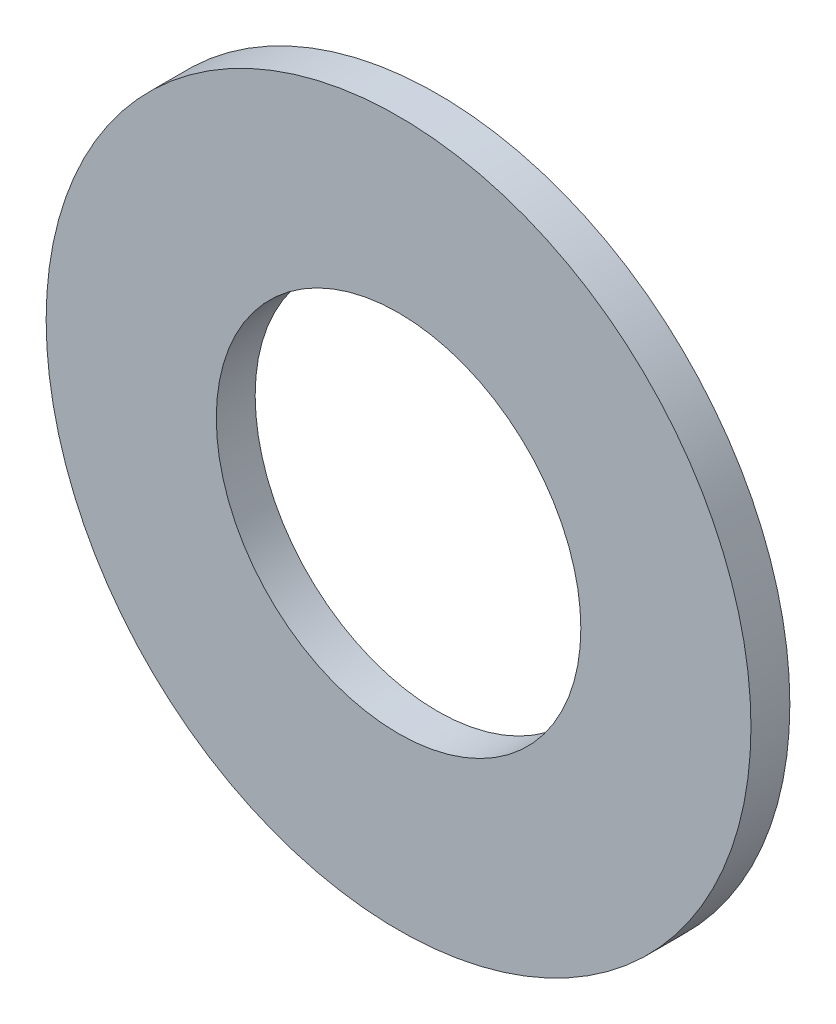
from build123d import *

# Parameters (mm, degrees)
SKETCH_1_R      = 29
SKETCH_1_R_2    = 15
EXTRUDE_1_DEPTH = 3.2


with BuildPart() as part:
    # 草图1 → 凸台-拉伸1 (new body)
    with BuildSketch(Plane.XY):
        Circle(SKETCH_1_R)
        Circle(SKETCH_1_R_2, mode=Mode.SUBTRACT)
    extrude(amount=EXTRUDE_1_DEPTH)


solid = part.part
